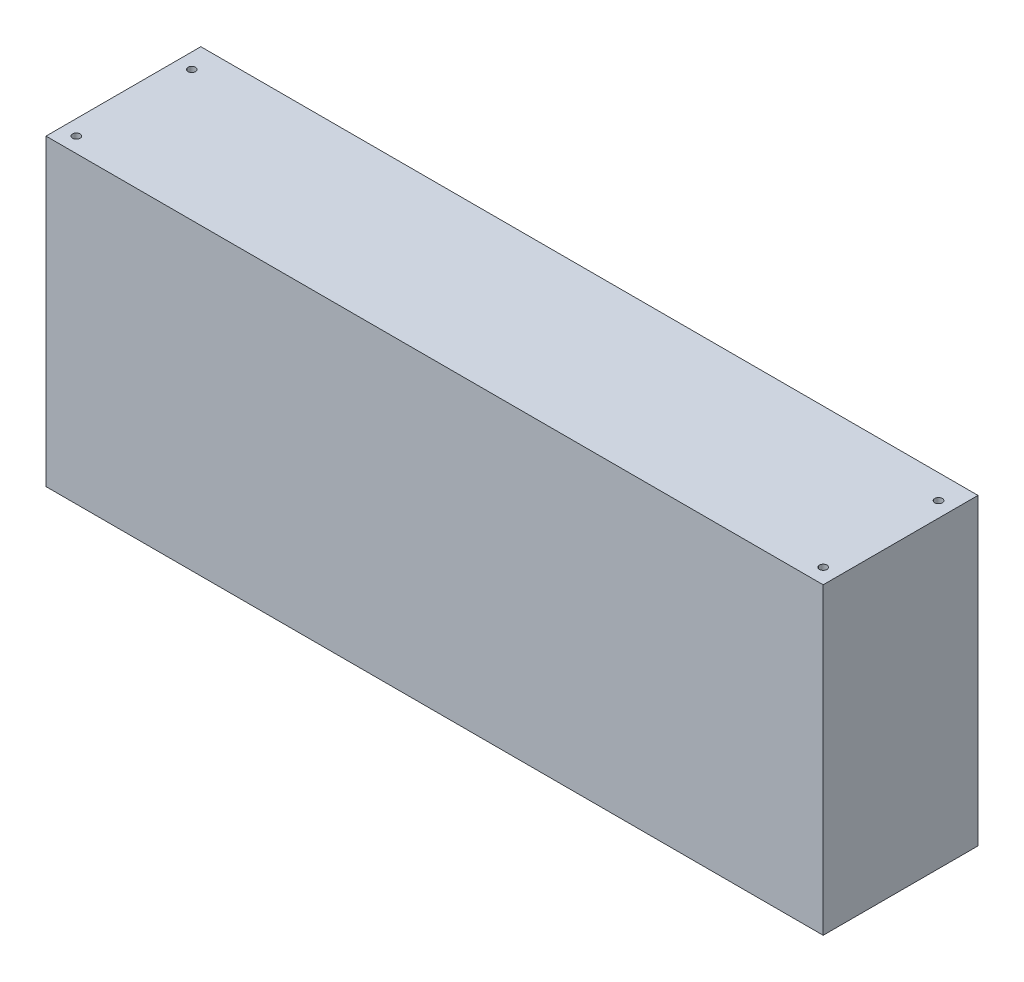
SolidWorks part; units mm, degrees
material "标准件"
ref_plane "前视基准面" through (0, 0, 0) normal (0, 0, 1) x (1, 0, 0)
ref_plane "上视基准面" through (0, 0, 0) normal (0, 1, 0) x (1, 0, 0)
ref_plane "右视基准面" through (0, 0, 0) normal (1, 0, 0) x (0, 0, -1)
sketch "草图1" plane through (0, 0, 0) normal (0, 0, 1) x (1, 0, 0)
  line L1 (-128, -50) -> (128, -50)
  line L2 (-128, -50) -> (-128, 50)
  line L3 (-128, 50) -> (128, 50)
  line L4 (128, -50) -> (128, 50)
  line L5 (-128, -50) -> (128, 50) construction
  line L6 (-128, 50) -> (128, -50) construction
  point P0 (0, 0)
  dimension "D1" = 100
  dimension "D2" = 256
extrude "凸台-拉伸1" add sketch "草图1" along normal mid plane 51
hole_wizard "M3 螺纹孔1" positions "草图2" profile "草图3" tap size "M3" standard "ISO"
sketch "草图2" plane through (0, 50, 0) normal (0, 1, 0) x (1, 0, 0)
  line L0 (0, 0) -> (0, 25.5) construction
  line L1 (128, 25.5) -> (-128, 25.5) construction
  line L3 (128, -25.5) -> (-128, -25.5) construction
  point P0 (-123, 17.5)
  point P2 (-123, -20.5)
  point P4 (123, 17.5)
  point P6 (123, -20.5)
  dimension "D1" = 5
  dimension "D2" = 38
  dimension "D3" = 246
sketch "草图3" plane through (-123, 50, -17.5) normal (1, 0, 0) x (0, 0, 1)
  line L0 (0, 0) -> (0, 8.2511)
  line L1 (0, 8.2511) -> (1.25, 7.5)
  line L2 (1.25, 7.5) -> (1.25, 0)
  line L5 (1.25, 0) -> (0, 0)
  line L10 (0, 8.2511) -> (-1.25, 7.5) construction
  line L11 (0, -6.35) -> (0, 107.95) construction
  dimension "螺纹孔钻头直径" = 2.5
  dimension "螺纹孔钻头深度" = 7.5
  dimension "导头角度" = 118
cosmetic thread "孔螺蚊线1"
cosmetic thread "孔螺蚊线2"
cosmetic thread "孔螺蚊线3"
cosmetic thread "孔螺蚊线4"
